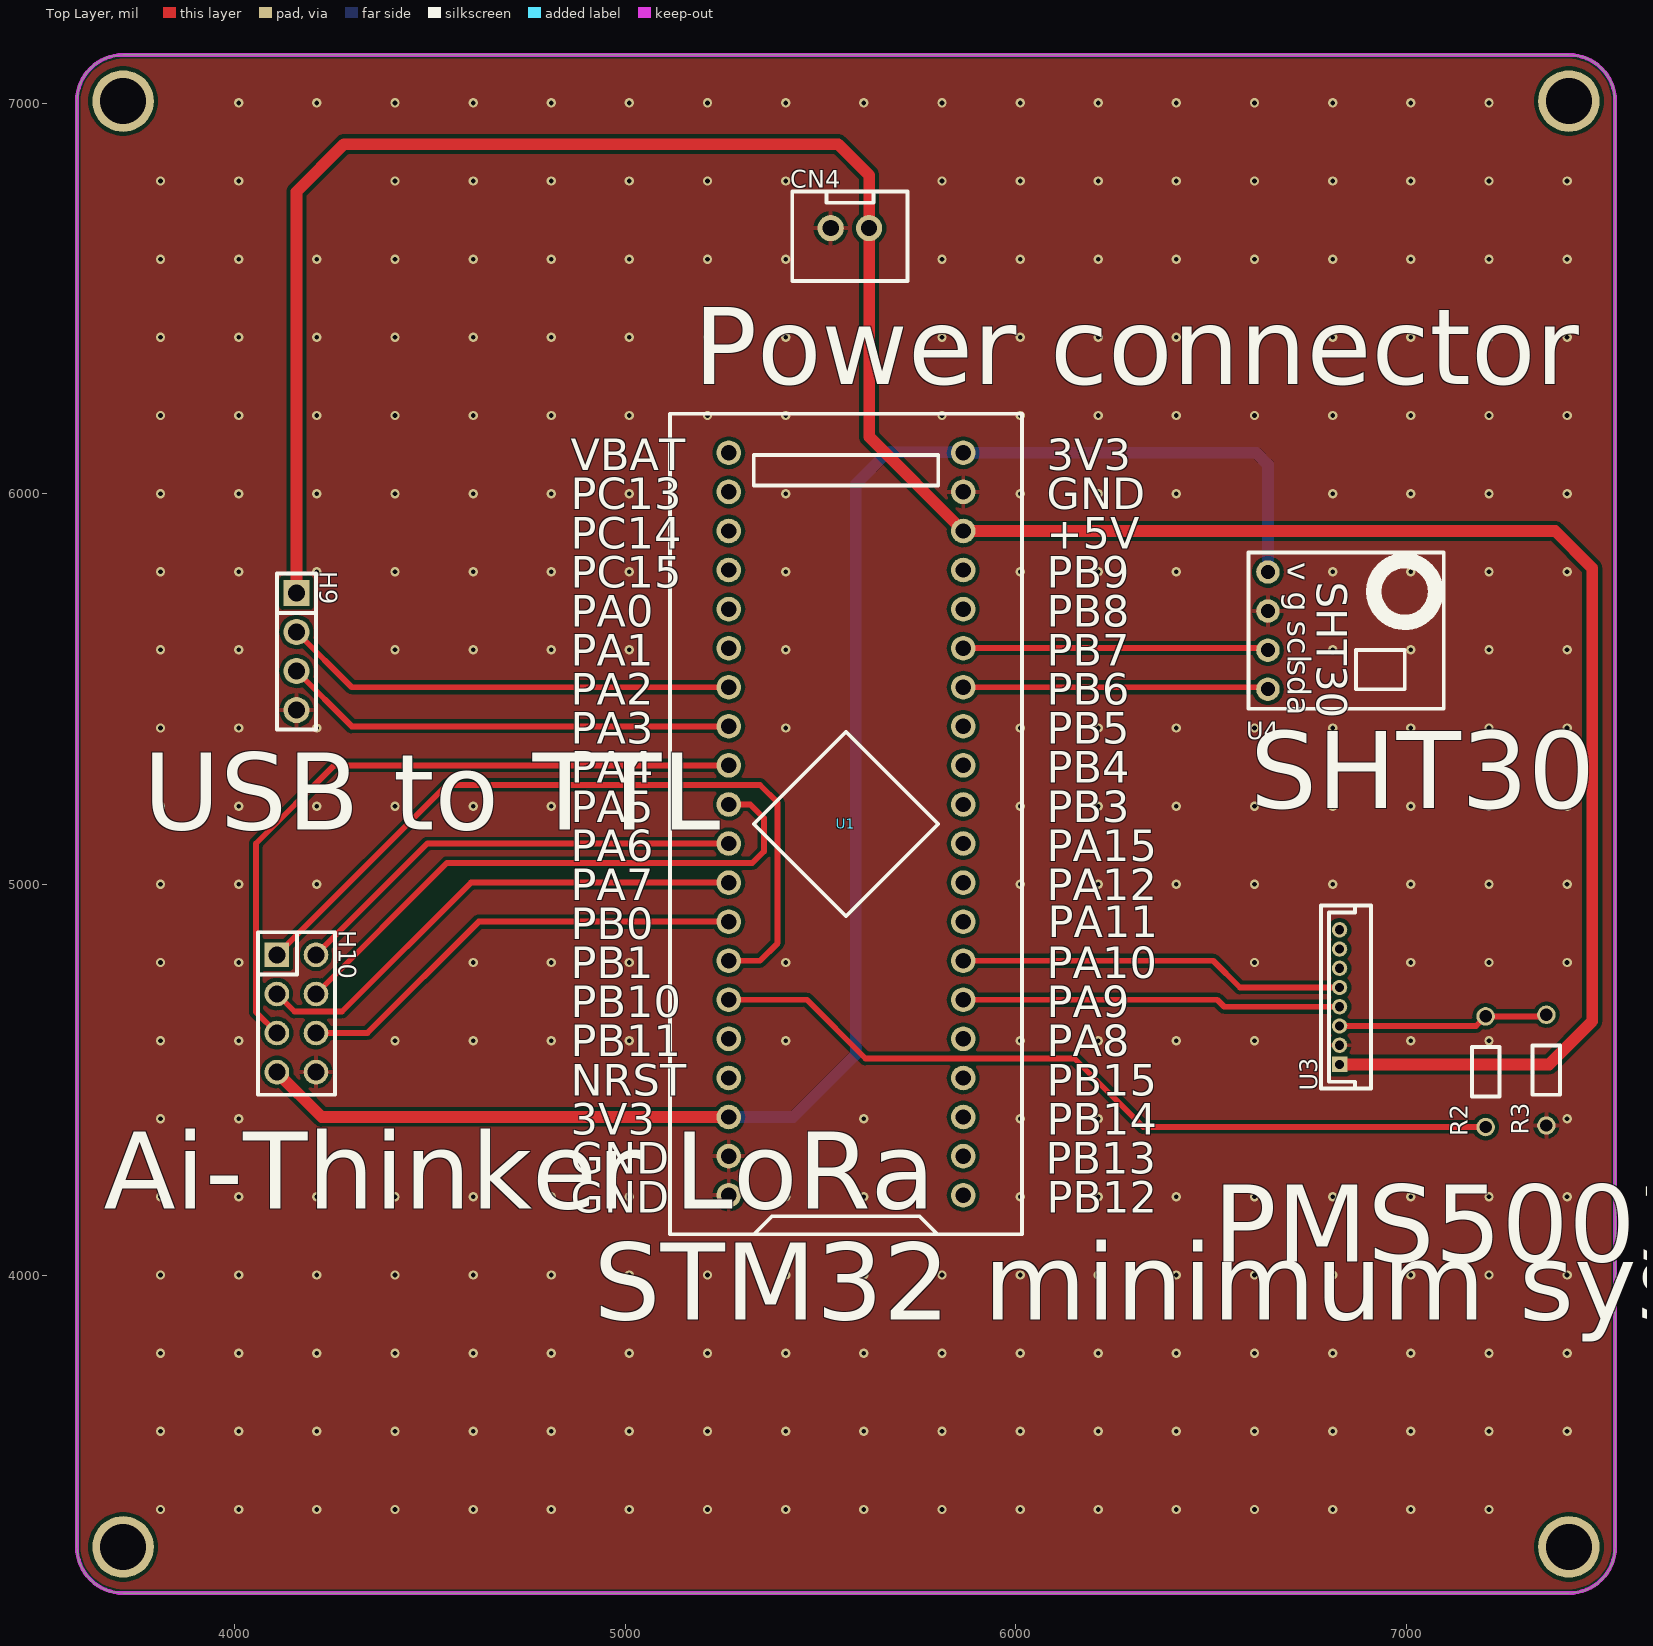
[diagram p0: Top Layer view]
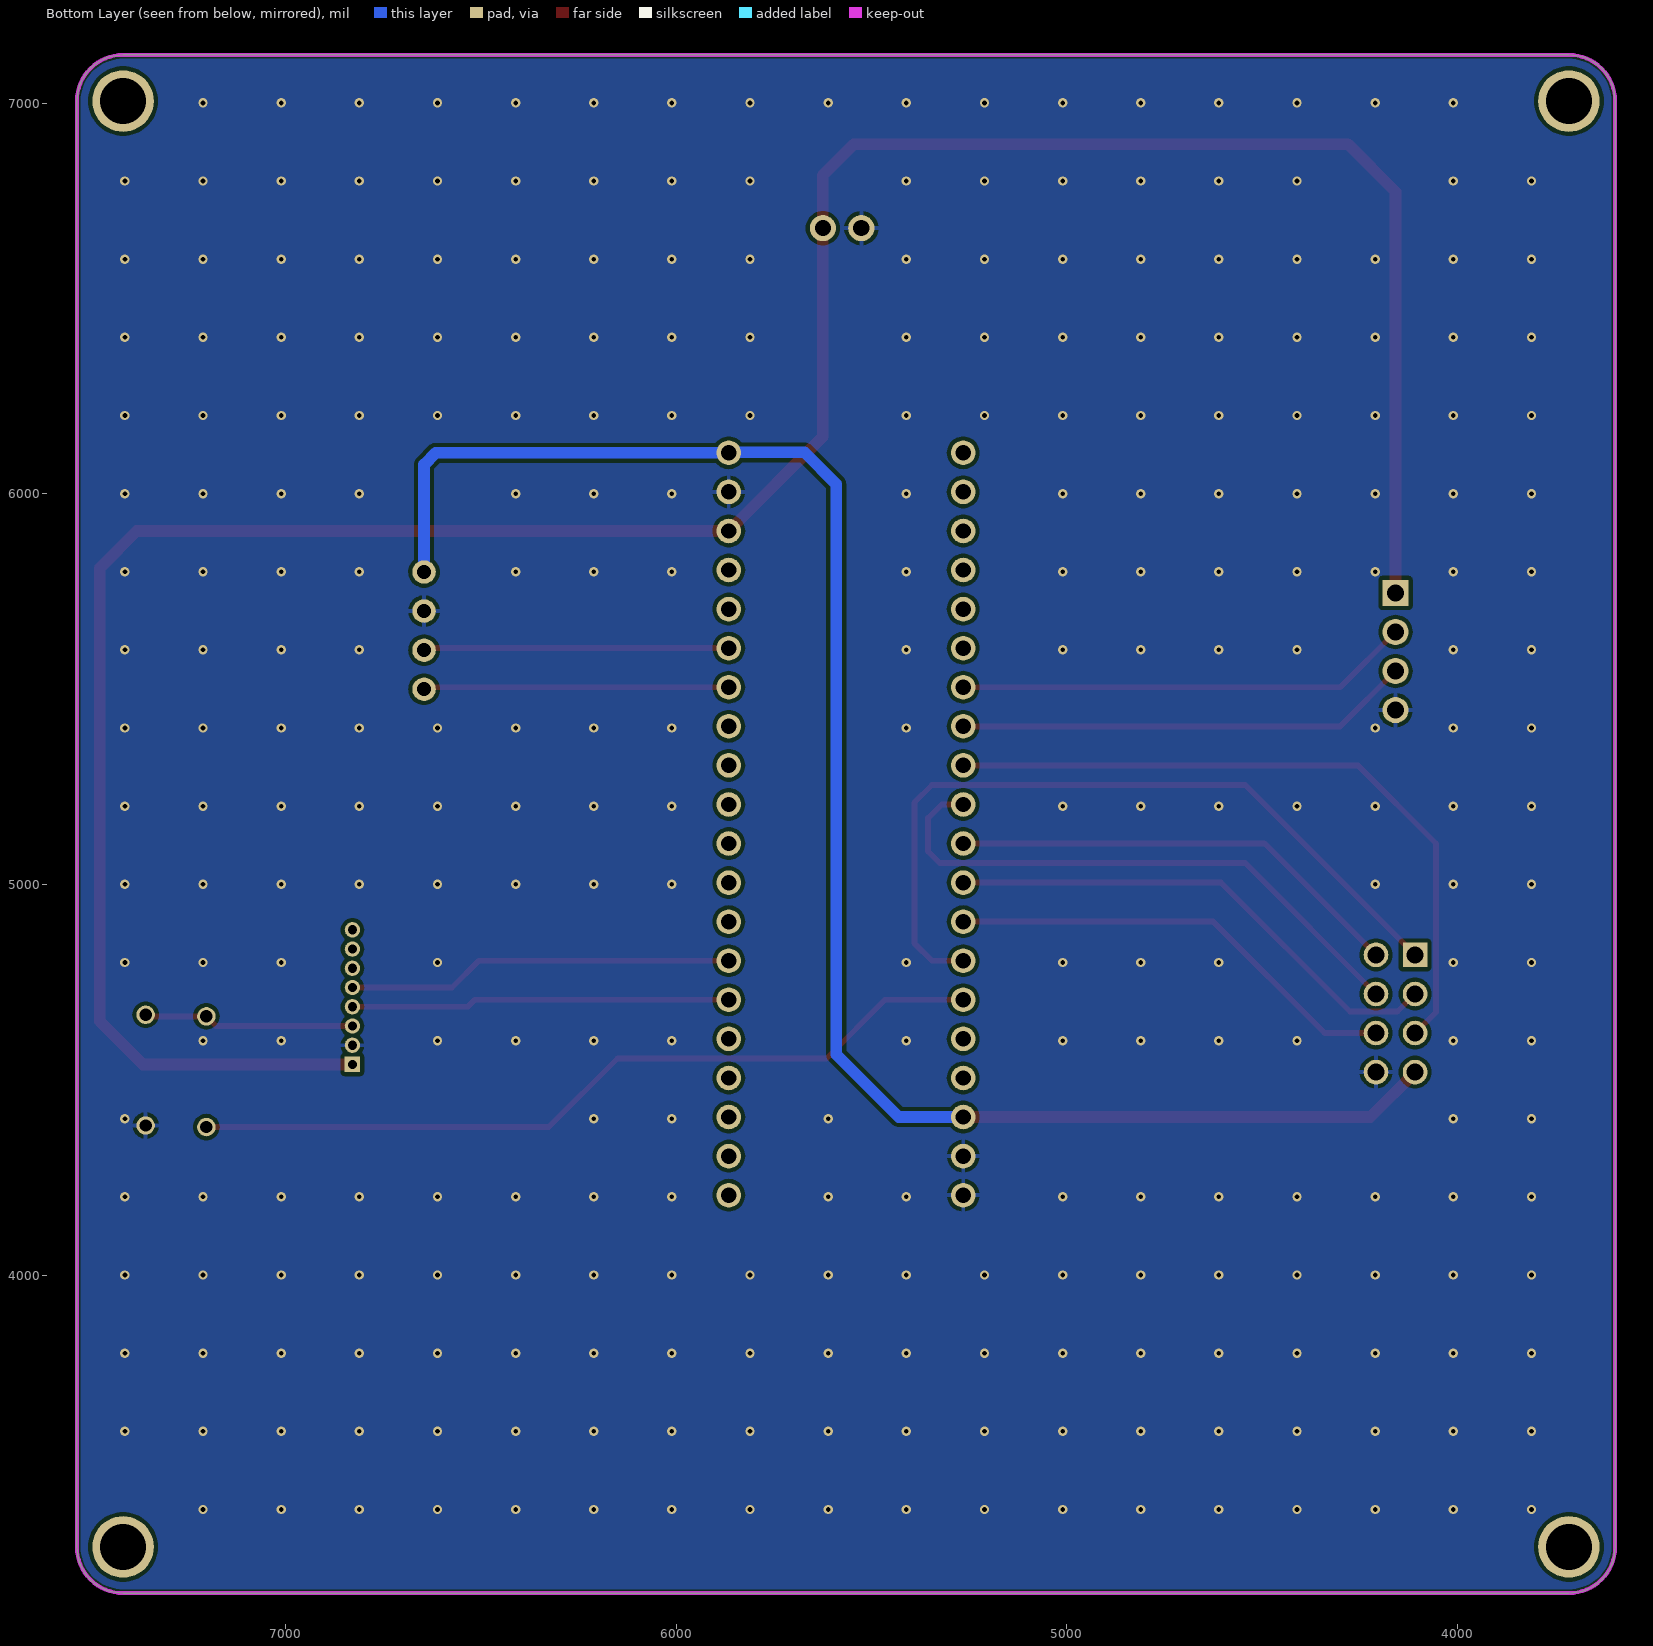
[diagram p1: Bottom Layer view, seen from below]
# Altium PCB MISC88998.pcbdoc
Units mil, origin at the board's own origin, x right, y up, seen from the top; angles counter-clockwise.
Board outline 3937.01 x 3937.01 mil, 2 copper layers (Top Layer, Bottom Layer), stack 62.206 mil thick; 8 components, 38 nets, 74 pads, 288 vias.

## Layer stack, top to bottom
Top Solder Mask Layer: solder mask 0.394, Dk 3.3
Top Layer: signal copper 1.379
Dielectric1: surface 59.449, FR4, Dk 4.5
Bottom Layer: signal copper 1.378
Bottom Solder Mask Layer: solder mask 0.394, Dk 3.3

## Board outline
3714.61,7123.5 ccw(c3714.61,7005.39) 3596.5,7005.39 3596.5,3304.61 ccw(c3714.61,3304.61) 3714.61,3186.5 7415.39,3186.5 ccw(c7415.39,3304.61) 7533.5,3304.61 7533.5,7005.39 ccw(c7415.39,7005.39) 7415.39,7123.5 3714.61,7123.5

## Design rules (kind name [scope] priority, off if disabled: settings)
BoardOutlineClearance copperThickness2oz_1 [All] p2 off: genericclearance=7.99 ignorepadtopadclearanceinfootprint=FALSE except(0: Arc-SplitContinuation Track-SplitContinuation SMDPad-SplitContinuation THPad-SplitContinuation Via-SplitContinuation Fill-SplitContinuation Region-SplitContinuation Poly-SplitContinuation Text-SplitContinuation Hole-SplitContinuation; 5.98: Arc-CutoutEdge Track-CutoutEdge SMDPad-CutoutEdge THPad-CutoutEdge Via-CutoutEdge Text-CutoutEdge; 6.9: Hole-OutlineEdge Hole-CutoutEdge; 10: Poly-OutlineEdge Poly-CutoutEdge; 11.81: Arc-OutlineEdge Track-OutlineEdge SMDPad-OutlineEdge THPad-OutlineEdge Via-OutlineEdge Fill-OutlineEdge Region-OutlineEdge Text-OutlineEdge Fill-CutoutEdge Region-CutoutEdge)
BoardOutlineClearance Plane_innerPlane_1 [All] p4 off: genericclearance=4.02 ignorepadtopadclearanceinfootprint=FALSE except(0: Arc-SplitContinuation Track-SplitContinuation SMDPad-SplitContinuation THPad-SplitContinuation Via-SplitContinuation Fill-SplitContinuation Region-SplitContinuation Poly-SplitContinuation Text-SplitContinuation Hole-SplitContinuation; 5.98: Arc-CutoutEdge Track-CutoutEdge SMDPad-CutoutEdge THPad-CutoutEdge Via-CutoutEdge Text-CutoutEdge; 6.9: Hole-OutlineEdge Hole-CutoutEdge; 10: Poly-OutlineEdge Poly-CutoutEdge; 11.81: Arc-OutlineEdge Track-OutlineEdge SMDPad-OutlineEdge THPad-OutlineEdge Via-OutlineEdge Fill-OutlineEdge Region-OutlineEdge Text-OutlineEdge Fill-CutoutEdge Region-CutoutEdge)
BoardOutlineClearance Copper_copperRegion_1 [All] p6 off: genericclearance=4.02 ignorepadtopadclearanceinfootprint=FALSE except(0: Arc-SplitContinuation Track-SplitContinuation SMDPad-SplitContinuation THPad-SplitContinuation Via-SplitContinuation Fill-SplitContinuation Region-SplitContinuation Poly-SplitContinuation Text-SplitContinuation Hole-SplitContinuation; 5.98: Arc-CutoutEdge Track-CutoutEdge SMDPad-CutoutEdge THPad-CutoutEdge Via-CutoutEdge Text-CutoutEdge; 6.9: Hole-OutlineEdge Hole-CutoutEdge; 10: Poly-OutlineEdge Poly-CutoutEdge; 11.81: Arc-OutlineEdge Track-OutlineEdge SMDPad-OutlineEdge THPad-OutlineEdge Via-OutlineEdge Fill-OutlineEdge Region-OutlineEdge Text-OutlineEdge Fill-CutoutEdge Region-CutoutEdge)
BoardOutlineClearance Copper_copperRegion_copperThickness1oz_1 [All] p8 off: genericclearance=4.02 ignorepadtopadclearanceinfootprint=FALSE except(0: Arc-SplitContinuation Track-SplitContinuation SMDPad-SplitContinuation THPad-SplitContinuation Via-SplitContinuation Fill-SplitContinuation Region-SplitContinuation Poly-SplitContinuation Text-SplitContinuation Hole-SplitContinuation; 5.98: Arc-CutoutEdge Track-CutoutEdge SMDPad-CutoutEdge THPad-CutoutEdge Via-CutoutEdge Text-CutoutEdge; 6.9: Hole-OutlineEdge Hole-CutoutEdge; 10: Poly-OutlineEdge Poly-CutoutEdge; 11.81: Arc-OutlineEdge Track-OutlineEdge SMDPad-OutlineEdge THPad-OutlineEdge Via-OutlineEdge Fill-OutlineEdge Region-OutlineEdge Text-OutlineEdge Fill-CutoutEdge Region-CutoutEdge)
BoardOutlineClearance Copper_copperRegion_Copper_copperRegion_1 [All] p10 off: genericclearance=4.02 ignorepadtopadclearanceinfootprint=FALSE except(0: Arc-SplitContinuation Track-SplitContinuation SMDPad-SplitContinuation THPad-SplitContinuation Via-SplitContinuation Fill-SplitContinuation Region-SplitContinuation Poly-SplitContinuation Text-SplitContinuation Hole-SplitContinuation; 5.98: Arc-CutoutEdge Track-CutoutEdge SMDPad-CutoutEdge THPad-CutoutEdge Via-CutoutEdge Text-CutoutEdge; 6.9: Hole-OutlineEdge Hole-CutoutEdge; 10: Poly-OutlineEdge Poly-CutoutEdge; 11.81: Arc-OutlineEdge Track-OutlineEdge SMDPad-OutlineEdge THPad-OutlineEdge Via-OutlineEdge Fill-OutlineEdge Region-OutlineEdge Text-OutlineEdge Fill-CutoutEdge Region-CutoutEdge)
BoardOutlineClearance copperThickness1oz_1 [All] p12: genericclearance=4.02 ignorepadtopadclearanceinfootprint=FALSE except(0: Arc-SplitContinuation Track-SplitContinuation SMDPad-SplitContinuation THPad-SplitContinuation Via-SplitContinuation Fill-SplitContinuation Region-SplitContinuation Poly-SplitContinuation Text-SplitContinuation Hole-SplitContinuation; 5.98: Arc-CutoutEdge Track-CutoutEdge SMDPad-CutoutEdge THPad-CutoutEdge Via-CutoutEdge Text-CutoutEdge; 6.9: Hole-OutlineEdge Hole-CutoutEdge; 10: Poly-OutlineEdge Poly-CutoutEdge; 11.81: Arc-OutlineEdge Track-OutlineEdge SMDPad-OutlineEdge THPad-OutlineEdge Via-OutlineEdge Fill-OutlineEdge Region-OutlineEdge Text-OutlineEdge Fill-CutoutEdge Region-CutoutEdge)
Clearance copperThickness2oz [All] p1 off: gap=7.99 ignorepadtopadclearanceinfootprint=FALSE except(5.98: SMDPad-Track SMDPad-SMDPad THPad-Track SMDPad-THPad THPad-THPad Track-Via SMDPad-Via THPad-Via Via-Via Fill-SMDPad Region-SMDPad Fill-THPad Region-THPad Fill-Via Region-Via Fill-Fill Fill-Region Region-Region Arc-Track Arc-SMDPad Arc-THPad Arc-Via Fill-Arc Region-Arc Arc-Arc Text-Track SMDPad-Text Text-THPad Text-Via Fill-Text Region-Text Arc-Text Text-Text; 6.9: Hole-Track Hole-SMDPad Hole-THPad Hole-Via Fill-Hole Region-Hole Hole-Arc Hole-Text; 10: Poly-Track Poly-SMDPad Poly-THPad Poly-Via Poly-Fill Poly-Region Poly-Poly Poly-Arc Poly-Text Poly-Hole; 11.81: Fill-Track Region-Track)
Clearance Plane_innerPlane [All] p3 off: gap=4.02 ignorepadtopadclearanceinfootprint=FALSE except(5.98: SMDPad-Track SMDPad-SMDPad THPad-Track SMDPad-THPad THPad-THPad Track-Via SMDPad-Via THPad-Via Via-Via Fill-SMDPad Region-SMDPad Fill-THPad Region-THPad Fill-Via Region-Via Fill-Fill Fill-Region Region-Region Arc-Track Arc-SMDPad Arc-THPad Arc-Via Fill-Arc Region-Arc Arc-Arc Text-Track SMDPad-Text Text-THPad Text-Via Fill-Text Region-Text Arc-Text Text-Text; 6.9: Hole-Track Hole-SMDPad Hole-THPad Hole-Via Fill-Hole Region-Hole Hole-Arc Hole-Text; 10: Poly-Track Poly-SMDPad Poly-THPad Poly-Via Poly-Fill Poly-Region Poly-Poly Poly-Arc Poly-Text Poly-Hole; 11.81: Fill-Track Region-Track)
Clearance Copper_copperRegion [All] p5 off: gap=4.02 ignorepadtopadclearanceinfootprint=FALSE except(5.98: SMDPad-Track SMDPad-SMDPad THPad-Track SMDPad-THPad THPad-THPad Track-Via SMDPad-Via THPad-Via Via-Via Fill-SMDPad Region-SMDPad Fill-THPad Region-THPad Fill-Via Region-Via Fill-Fill Fill-Region Region-Region Arc-Track Arc-SMDPad Arc-THPad Arc-Via Fill-Arc Region-Arc Arc-Arc Text-Track SMDPad-Text Text-THPad Text-Via Fill-Text Region-Text Arc-Text Text-Text; 6.9: Hole-Track Hole-SMDPad Hole-THPad Hole-Via Fill-Hole Region-Hole Hole-Arc Hole-Text; 10: Poly-Track Poly-SMDPad Poly-THPad Poly-Via Poly-Fill Poly-Region Poly-Poly Poly-Arc Poly-Text Poly-Hole; 11.81: Fill-Track Region-Track)
Clearance Copper_copperRegion_copperThickness1oz [All] p7 off: gap=4.02 ignorepadtopadclearanceinfootprint=FALSE except(5.98: SMDPad-Track SMDPad-SMDPad THPad-Track SMDPad-THPad THPad-THPad Track-Via SMDPad-Via THPad-Via Via-Via Fill-SMDPad Region-SMDPad Fill-THPad Region-THPad Fill-Via Region-Via Fill-Fill Fill-Region Region-Region Arc-Track Arc-SMDPad Arc-THPad Arc-Via Fill-Arc Region-Arc Arc-Arc Text-Track SMDPad-Text Text-THPad Text-Via Fill-Text Region-Text Arc-Text Text-Text; 6.9: Hole-Track Hole-SMDPad Hole-THPad Hole-Via Fill-Hole Region-Hole Hole-Arc Hole-Text; 10: Poly-Track Poly-SMDPad Poly-THPad Poly-Via Poly-Fill Poly-Region Poly-Poly Poly-Arc Poly-Text Poly-Hole; 11.81: Fill-Track Region-Track)
Clearance Copper_copperRegion_Copper_copperRegion [All] p9 off: gap=4.02 ignorepadtopadclearanceinfootprint=FALSE except(5.98: SMDPad-Track SMDPad-SMDPad THPad-Track SMDPad-THPad THPad-THPad Track-Via SMDPad-Via THPad-Via Via-Via Fill-SMDPad Region-SMDPad Fill-THPad Region-THPad Fill-Via Region-Via Fill-Fill Fill-Region Region-Region Arc-Track Arc-SMDPad Arc-THPad Arc-Via Fill-Arc Region-Arc Arc-Arc Text-Track SMDPad-Text Text-THPad Text-Via Fill-Text Region-Text Arc-Text Text-Text; 6.9: Hole-Track Hole-SMDPad Hole-THPad Hole-Via Fill-Hole Region-Hole Hole-Arc Hole-Text; 10: Poly-Track Poly-SMDPad Poly-THPad Poly-Via Poly-Fill Poly-Region Poly-Poly Poly-Arc Poly-Text Poly-Hole; 11.81: Fill-Track Region-Track)
Clearance copperThickness1oz [All] p11: gap=4.02 ignorepadtopadclearanceinfootprint=FALSE except(5.98: SMDPad-Track SMDPad-SMDPad THPad-Track SMDPad-THPad THPad-THPad Track-Via SMDPad-Via THPad-Via Via-Via Fill-SMDPad Region-SMDPad Fill-THPad Region-THPad Fill-Via Region-Via Fill-Fill Fill-Region Region-Region Arc-Track Arc-SMDPad Arc-THPad Arc-Via Fill-Arc Region-Arc Arc-Arc Text-Track SMDPad-Text Text-THPad Text-Via Fill-Text Region-Text Arc-Text Text-Text; 6.9: Hole-Track Hole-SMDPad Hole-THPad Hole-Via Fill-Hole Region-Hole Hole-Arc Hole-Text; 10: Poly-Track Poly-SMDPad Poly-THPad Poly-Via Poly-Fill Poly-Region Poly-Poly Poly-Arc Poly-Text Poly-Hole; 11.81: Fill-Track Region-Track)
DiffPairsRouting differentialPair [All] p1: maxlimit=6 minlimit=6 mostfreqgap=6 toplayer_minwidth=5 toplayer_prefwidth=10 toplayer_maxwidth=100 toplayer_mingap=6 toplayer_prefgap=6 toplayer_maxgap=6 bottomlayer_minwidth=5 bottomlayer_prefwidth=10 bottomlayer_maxwidth=100 bottomlayer_mingap=6 bottomlayer_prefgap=6 bottomlayer_maxgap=6 maxuncoupledlength=10
HoleToHoleClearance otherClearance [All] p1: gap=11.81 allowstackedmicrovias=TRUE
Length netLength [All] p1: minlimit=0 maxlimit=0
PasteMaskExpansion pasteMaskExpansion [All] p1: expansion=0
PlaneConnect innerPlane [All] p1: planeconnectstyle=Relief reliefexpansion=20 reliefentries=4 reliefconductorwidth=10 reliefairgap=10
PolygonConnect copperRegion_copperThickness1oz [All] p1 off: connectstyle=Relief reliefconductorwidth=10 reliefentries=4 polygonreliefangle="90 Angle" airgapwidth=10 via.connectstyle=Relief via.reliefconductorwidth=10 via.reliefentries=4 via.polygonreliefangle="90 Angle" via.airgapwidth=10
PolygonConnect copperRegion_Copper_copperRegion [All] p2 off: connectstyle=Relief reliefconductorwidth=10 reliefentries=4 polygonreliefangle="90 Angle" airgapwidth=10 via.connectstyle=Relief via.reliefconductorwidth=10 via.reliefentries=4 via.polygonreliefangle="90 Angle" via.airgapwidth=10
PolygonConnect copperRegion [All] p3: connectstyle=Relief reliefconductorwidth=10 reliefentries=4 polygonreliefangle="90 Angle" airgapwidth=10 via.connectstyle=Relief via.reliefconductorwidth=10 via.reliefentries=4 via.polygonreliefangle="90 Angle" via.airgapwidth=10
RoutingVias viaSize [All] p1: holewidth=12.01 width=24.02 viastyle="Through Hole" minholewidth=11.81 minwidth=19.68 maxholewidth=248.03 maxwidth=393.7
SolderMaskExpansion solderMaskExpansion [IsVia] p1: expansion=-1000 istentingtop=TRUE
SolderMaskExpansion solderMaskExpansion [All] p2: expansion=2 istentingtop=FALSE
Width copperThickness2oz_2 [All] p1 off: maxlimit=100 minlimit=8 preferedwidth=10
Width copperThickness1oz_2 [All] p2: maxlimit=100 minlimit=5 preferedwidth=10

## Components (designator, comment, footprint, x,y, rotation, side; value= is the part's Value field where it differs from the comment)
CN4 "XH2.54*2P_THT" CONN-TH_2P-P2.50-XH2.54-2P 5575,6680 r0 top
H9 "" HDR-TH_4P-P2.54-V-M 4158.51,5596.46 r270 top
H10 "" HDR-TH_8P-P2.54-V-F-R2-C4-S2.54-1 4158.51,4670 r270 top
R2 "1kΩ" Res_1/8W 7204.63,4520.95 r90 top
R3 "10kΩ" Res_1/8W 7360,4525 r90 top
U1 "STM32F103C8T6-Card" CONN-TH_L53.3-W22.9_STM32F103C8T6-CARD 5565,5155 r90 top
U3 "PMS5003" 1.25-LI-8P 6828.27,4711.85 r90 top
U4 "" SHT30模块 6845,5650 r0 top

## Footprints (in the part's own frame and the unit in brackets; to place one, negate y for a bottom-side part, rotate by r counter-clockwise, add the part's x,y. Pads: shape width x height; smd on the part's side, far side on the other; paste and mask are expansions set on the pad)
1.25-LI-8P [mm]
  rect 1x1 hole 0.6 paste+0 mask+0.05: 1(-4.375,0)
  round 1 hole 0.6 paste+0 mask+0.05: 2(-3.125,0) 5(0.625,0) 6(1.875,0)
  round 1 hole 0.6 copper offset 0,0 paste+0 mask+0.05: 3(-1.875,0) 4(-0.625,0) 7(3.125,0) 8(4.375,0)
  silkscreen extent -5.95,-2.05 5.95,1.2
CONN-TH_2P-P2.50-XH2.54-2P [mm]
  round 1.7 hole 1.05 paste+0 mask+0.05: 1(1.25,0) 2(-1.25,0)
  silkscreen extent -3.75,-3.42 3.75,2.37
CONN-TH_L53.3-W22.9_STM32F103C8T6-CARD [mm]
  round 1.6 hole 1: 1(-24.13,-7.62) 2(-21.59,-7.62) 3(-19.05,-7.62) 4(-16.51,-7.62) 5(-13.97,-7.62) 6(-11.43,-7.62) 7(-8.89,-7.62) 8(-6.35,-7.62) 9(-3.81,-7.62) 10(-1.27,-7.62) 11(1.27,-7.62) 12(3.81,-7.62) 13(6.35,-7.62) 14(8.89,-7.62) 15(11.43,-7.62) 16(13.97,-7.62) 17(16.51,-7.62) 18(19.05,-7.62) 19(21.59,-7.62) 20(24.13,-7.62) 21(24.13,7.62) 22(21.59,7.62) 23(19.05,7.62) 24(16.51,7.62) 25(13.97,7.62) 26(11.43,7.62) 27(8.89,7.62) 28(6.35,7.62) 29(3.81,7.62) 30(1.27,7.62) 31(-1.27,7.62) 32(-3.81,7.62) 33(-6.35,7.62) 34(-8.89,7.62) 35(-11.43,7.62) 36(-13.97,7.62) 37(-16.51,7.62) 38(-19.05,7.62) 39(-21.59,7.62) 40(-24.13,7.62)
  silkscreen extent -26.67,-11.43 26.67,11.43
HDR-TH_4P-P2.54-V-M [mm]
  rect 1.7x1.7 hole 1.1: 1(-3.81,0)
  round 1.7 hole 1.1: 2(-1.27,0) 3(1.27,0) 4(3.81,0)
  silkscreen extent -5.08,-1.27 5.08,1.27
HDR-TH_8P-P2.54-V-F-R2-C4-S2.54-1 [mm]
  rect 1.6x1.6 hole 1.1: 1(-3.81,-1.27)
  round 1.6 hole 1.1: 2(-3.81,1.27) 3(-1.27,-1.27) 4(-1.27,1.27) 5(1.27,-1.27) 6(1.27,1.27) 7(3.81,-1.27) 8(3.81,1.27)
  silkscreen extent -5.28,-2.5 5.28,2.5
Res_1/8W [mil]
  round 47.2 hole 31.5 paste+0 mask+2: 1(-141.7,2.48) 2(141.7,2.48)
  silkscreen extent -63,-33 63,38
SHT30模块 [mil]
  round 60 hole 36 paste+0 mask+4: 1(-200,150) 2(-200,50) 3(-200,-50) 4(-200,-150)
  silkscreen extent -250,-200 250,200

## Free pads (board coordinates)
  round 157.48 hole 118.11: 1(3714.61,7005.39) 1(3714.61,3304.61) 1(7415.39,7005.39) 1(7415.39,3304.61)

## Via types
v1: diameter 24.02, hole 12, Top Layer to Bottom Layer, 288 vias

## Nets (pads, with @x,y where several pads share a name; then routed paths per layer and width w, separated by ;. In a path a pad name is that pad's centre, name@x,y a point inside that pad or via, vN(x,y) a via of type N, cw(c..) or ccw(c..) an arc to the next point about the centre after c; other vN are vias at no path point)
$1N17264: R2.2 R3.2 U3.3 | length 541.1
  Top Layer w15: U3.3 7177.55,4638.04 R2.2 7353.47,4662.65 R3.2
+5V: CN4.1 H9.1 U1.18 U3.1 | length 7088.2
  Top Layer w30: H9.1 4158.51,6773.51 4280,6895 5545,6895 5624.22,6815.78 CN4.1 5624.22,6145.79 U1.18 7380,5905 7475,5810 7475,4650 7364.61,4539.61 U3.1
GND: CN4.2 H9.4 H10.8 R3.1 U1.19 U1.39 U1.40 U3.2 U4.2
  other v1: 3810.6,3400.6 4010.6,3400.6 4210.6,3400.6 4410.6,3400.6 4610.6,3400.6 4810.6,3400.6 5010.6,3400.6 5210.6,3400.6 5410.6,3400.6 5610.6,3400.6 5810.6,3400.6 6010.6,3400.6 6210.6,3400.6 6410.6,3400.6 6610.6,3400.6 6810.6,3400.6 7010.6,3400.6 7210.6,3400.6 3810.6,3600.6 4010.6,3600.6 4210.6,3600.6 4410.6,3600.6 4610.6,3600.6 4810.6,3600.6 5010.6,3600.6 5210.6,3600.6 5410.6,3600.6 5610.6,3600.6 5810.6,3600.6 6010.6,3600.6 6210.6,3600.6 6410.6,3600.6 6610.6,3600.6 6810.6,3600.6 7010.6,3600.6 7210.6,3600.6 7410.6,3600.6 3810.6,3800.6 4010.6,3800.6 4210.6,3800.6 4410.6,3800.6 4610.6,3800.6 4810.6,3800.6 5010.6,3800.6 5210.6,3800.6 5410.6,3800.6 5610.6,3800.6 5810.6,3800.6 6010.6,3800.6 6210.6,3800.6 6410.6,3800.6 6610.6,3800.6 6810.6,3800.6 7010.6,3800.6 7210.6,3800.6 7410.6,3800.6 3810.6,4000.6 4010.6,4000.6 4210.6,4000.6 4410.6,4000.6 4610.6,4000.6 4810.6,4000.6 5010.6,4000.6 5210.6,4000.6 5410.6,4000.6 5610.6,4000.6 5810.6,4000.6 6010.6,4000.6 6210.6,4000.6 6410.6,4000.6 6610.6,4000.6 6810.6,4000.6 7010.6,4000.6 7210.6,4000.6 7410.6,4000.6 3810.6,4200.6 4010.6,4200.6 4210.6,4200.6 4410.6,4200.6 4610.6,4200.6 4810.6,4200.6 5010.6,4200.6 5410.6,4200.6 5610.6,4200.6 6010.6,4200.6 6210.6,4200.6 6410.6,4200.6 6610.6,4200.6 6810.6,4200.6 7010.6,4200.6 7210.6,4200.6 7410.6,4200.6 3810.6,4400.6 4010.6,4400.6 5610.6,4400.6 6010.6,4400.6 6210.6,4400.6 7410.6,4400.6 3810.6,4600.6 4010.6,4600.6 4410.6,4600.6 4610.6,4600.6 4810.6,4600.6 5010.6,4600.6 5410.6,4600.6 6010.6,4600.6 6210.6,4600.6 6410.6,4600.6 6610.6,4600.6 7010.6,4600.6 7210.6,4600.6 3810.6,4800.6 4010.6,4800.6 4610.6,4800.6 4810.6,4800.6 5010.6,4800.6 5410.6,4800.6 6610.6,4800.6 7010.6,4800.6 7210.6,4800.6 7410.6,4800.6 3810.6,5000.6 4010.6,5000.6 4210.6,5000.6 6010.6,5000.6 6210.6,5000.6 6410.6,5000.6 6610.6,5000.6 6810.6,5000.6 7010.6,5000.6 7210.6,5000.6 7410.6,5000.6 3810.6,5200.6 4010.6,5200.6 4210.6,5200.6 4410.6,5200.6 4610.6,5200.6 4810.6,5200.6 5010.6,5200.6 6010.6,5200.6 6210.6,5200.6 6410.6,5200.6 6610.6,5200.6 6810.6,5200.6 7010.6,5200.6 7210.6,5200.6 7410.6,5200.6 3810.6,5400.6 4010.6,5400.6 4210.6,5400.6 5410.6,5400.6 6010.6,5400.6 6210.6,5400.6 6410.6,5400.6 6610.6,5400.6 6810.6,5400.6 7010.6,5400.6 7210.6,5400.6 7410.6,5400.6 3810.6,5600.6 4010.6,5600.6 4410.6,5600.6 4610.6,5600.6 4810.6,5600.6 5010.6,5600.6 5410.6,5600.6 6810.6,5600.6 7010.6,5600.6 7210.6,5600.6 7410.6,5600.6 3810.6,5800.6 4010.6,5800.6 4210.6,5800.6 4410.6,5800.6 4610.6,5800.6 4810.6,5800.6 5010.6,5800.6 5410.6,5800.6 6010.6,5800.6 6210.6,5800.6 6410.6,5800.6 6810.6,5800.6 7010.6,5800.6 7210.6,5800.6 7410.6,5800.6 3810.6,6000.6 4010.6,6000.6 4210.6,6000.6 4410.6,6000.6 4610.6,6000.6 4810.6,6000.6 5010.6,6000.6 5410.6,6000.6 6010.6,6000.6 6210.6,6000.6 6410.6,6000.6 6810.6,6000.6 7010.6,6000.6 7210.6,6000.6 7410.6,6000.6 3810.6,6200.6 4010.6,6200.6 4210.6,6200.6 4410.6,6200.6 4610.6,6200.6 4810.6,6200.6 5010.6,6200.6 5210.6,6200.6 5410.6,6200.6 5810.6,6200.6 6010.6,6200.6 6210.6,6200.6 6410.6,6200.6 6610.6,6200.6 6810.6,6200.6 7010.6,6200.6 7210.6,6200.6 7410.6,6200.6 3810.6,6400.6 4010.6,6400.6 4210.6,6400.6 4410.6,6400.6 4610.6,6400.6 4810.6,6400.6 5010.6,6400.6 5210.6,6400.6 5410.6,6400.6 5810.6,6400.6 6010.6,6400.6 6210.6,6400.6 6410.6,6400.6 6610.6,6400.6 6810.6,6400.6 7010.6,6400.6 7210.6,6400.6 7410.6,6400.6 3810.6,6600.6 4010.6,6600.6 4210.6,6600.6 4410.6,6600.6 4610.6,6600.6 4810.6,6600.6 5010.6,6600.6 5210.6,6600.6 5410.6,6600.6 5810.6,6600.6 6010.6,6600.6 6210.6,6600.6 6410.6,6600.6 6610.6,6600.6 6810.6,6600.6 7010.6,6600.6 7210.6,6600.6 7410.6,6600.6 3810.6,6800.6 4010.6,6800.6 4410.6,6800.6 4610.6,6800.6 4810.6,6800.6 5010.6,6800.6 5210.6,6800.6 5410.6,6800.6 5810.6,6800.6 6010.6,6800.6 6210.6,6800.6 6410.6,6800.6 6610.6,6800.6 6810.6,6800.6 7010.6,6800.6 7210.6,6800.6 7410.6,6800.6 4010.6,7000.6 4210.6,7000.6 4410.6,7000.6 4610.6,7000.6 4810.6,7000.6 5010.6,7000.6 5210.6,7000.6 5410.6,7000.6 5610.6,7000.6 5810.6,7000.6 6010.6,7000.6 6210.6,7000.6 6410.6,7000.6 6610.6,7000.6 6810.6,7000.6 7010.6,7000.6 7210.6,7000.6
NRST: U1.37
PA0: U1.25
PA1: U1.26
PA2: H9.2 U1.27 | length 1165.1
  Top Layer w15: H9.2 4299.97,5505 U1.27
PA3: H9.3 U1.28 | length 1165.1
  Top Layer w15: H9.3 4299.97,5405 U1.28
PA4: H10.5 U1.29 | length 1800
  Top Layer w15: H10.5 4055,4673.51 4055,5105 4255,5305 U1.29
PA5: H10.4 U1.30 | length 1487.2
  Top Layer w15: H10.4 4543.51,5055 5325,5055 5355,5085 5355,5170 5320,5205 U1.30
PA6: H10.2 U1.31 | length 1174.5
  Top Layer w15: H10.2 4493.51,5105 U1.31
PA7: H10.3 U1.32 | length 1311.8
  Top Layer w15: H10.3 4153.51,4675 4275,4675 4605,5005 U1.32
PA8: U1.5
PA9: U1.6 U3.4 | length 970.6
  Top Layer w15: U1.6 6515,4705 6532.75,4687.25 U3.4
PA10: U1.7 U3.5 | length 991.7
  Top Layer w15: U1.7 6505,4805 6573.54,4736.46 U3.5
PA11: U1.8
PA12: U1.9
PA15: U1.10
PB0: H10.6 U1.33 | length 1174.5
  Top Layer w15: H10.6 4340,4620 4625,4905 U1.33
PB1: H10.1 U1.34 | length 1984
  Top Layer w15: H10.1 4543.51,5255 5345,5255 5390,5210 5390,4850 5345,4805 U1.34
PB3: U1.11
PB4: U1.12
PB5: U1.13
PB6: U1.14 U4.4 | length 782.1
  Top Layer w15: U1.14 6640,5505 U4.4
PB7: U1.15 U4.3 | length 782.1
  Top Layer w15: U1.15 6640,5605 U4.3
PB8: U1.16
PB9: U1.17
PB10: R2.1 U1.35 | length 2072.1
  Top Layer w15: U1.35 5465,4705 5615,4555 6150,4555 6325.75,4379.25 R2.1
PB11: U1.36
PB12: U1.1
PB13: U1.2
PB14: U1.3
PB15: U1.4
PC13: U1.22
PC14: U1.23
PC15: U1.24
VBAT: U1.21
VCC: H10.7 U1.20 U1.38 U4.1 | length 4432
  Top Layer w30: H10.7 4223.51,4405 U1.38
  Bottom Layer w30: U1.38 5430,4405 5590,4565 5590,6025 5671.21,6106.21 5863.79,6106.21 U1.20 6615,6105 6645,6075 U4.1
pads on no net: U3.6 U3.7 U3.8

## Polygon pours and split planes (outlines as drawn)
GND on Bottom Layer (solid, remove dead copper, pour order 2): 3525,7245 3525,3080 7700,3080 7700,7245
GND on Top Layer (solid, remove dead copper, pour order 2): 3000,7415 3000,3000 7930,3000 7930,7415

## Keep-outs
Board Outline Layer:
  the board outline again, w10

## Silkscreen, mask and mechanical layers (free items; w line width, h text height)
Top Silkscreen Layer:
  text "Power connector" at 5175,6280 h196.85
  text "VBAT" at 4860.95,6060 h80
  text "3V3" at 6079.16,6060 h80
  text "PC13" at 4860.95,5960 h80
  text "GND" at 6079.16,5960 h80
  text "PC14" at 4860.95,5860 h80
  text "+5V" at 6079.16,5860 h80
  text "PC15" at 4860.95,5760 h80
  text "PB9" at 6079.16,5760 h80
  text "PA0" at 4860.95,5660 h80
  text "PB8" at 6079.16,5660 h80
  text "PA1" at 4860.95,5560 h80
  text "PB7" at 6079.16,5560 h80
  text "PA2" at 4860.95,5460 h80
  text "PB6" at 6079.16,5460 h80
  text "PA3" at 4860.95,5360 h80
  text "PB5" at 6079.16,5360 h80
  text "PA4" at 4860.95,5260 h80
  text "PB4" at 6079.16,5260 h80
  text "SHT30" at 6599.83,5195 h196.85
  text "PA5" at 4860.95,5160 h80
  text "PB3" at 6079.16,5160 h80
  text "USB to TTL" at 3766.75,5140 h196.85
  text "PA6" at 4860.95,5060 h80
  text "PA15" at 6079.16,5060 h80
  text "PA7" at 4860.95,4960 h80
  text "PA12" at 6079.16,4960 h80
  text "PA11" at 6080.95,4865 h80
  text "PB0" at 4860.95,4860 h80
  text "PB1" at 4860.95,4760 h80
  text "PA10" at 6079.16,4760 h80
  text "PB10" at 4860.95,4660 h80
  text "PA9" at 6079.16,4660 h80
  text "PB11" at 4860.95,4560 h80
  text "PA8" at 6079.16,4560 h80
  text "NRST" at 4860.95,4460 h80
  text "PB15" at 6079.16,4460 h80
  text "3V3" at 4860.95,4360 h80
  text "PB14" at 6079.16,4360 h80
  text "GND" at 4860.95,4260 h80
  text "PB13" at 6075.95,4260 h80
  text "Ai-Thinker LoRa" at 3665.64,4170 h196.85
  text "GND" at 4860.95,4160 h80
  text "PB12" at 6079.16,4160 h80
  text "PMS5003" at 6504.69,4035 h196.85
  text "STM32 minimum system" at 4919.45,3886.57 h196.85